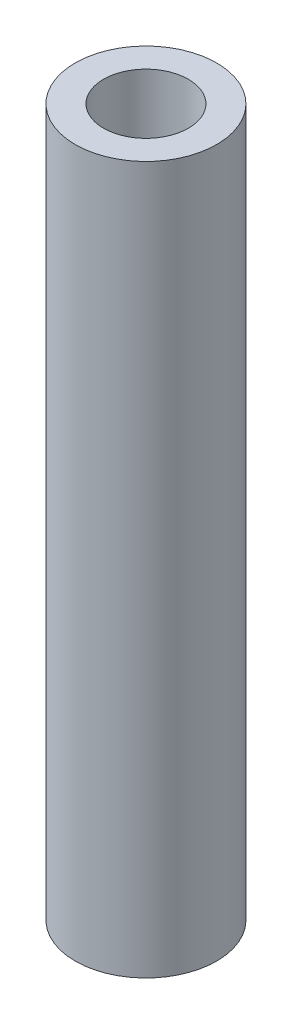
from build123d import *

# Parameters (mm, degrees)
SKETCH1_R           = 2.5
SKETCH1_R_2         = 1.5
BOSS_EXTRUDE1_DEPTH = 25
SKETCH2_R           = 1.5
SKETCH2_R_2         = 0.5
BOSS_EXTRUDE2_DEPTH = 2


with BuildPart() as part:
    # Sketch1 → Boss-Extrude1 (new body)
    with BuildSketch(Plane(origin=(0, 0, 0), x_dir=(1, 0, 0), z_dir=(0, 1, 0))):
        with Locations(Location((0, 0, 0), (0, 0, 270))):
            Circle(SKETCH1_R)
        with Locations(Location((0, 0, 0), (0, 0, 270))):
            Circle(SKETCH1_R_2, mode=Mode.SUBTRACT)
    extrude(amount=BOSS_EXTRUDE1_DEPTH)

    # Sketch2 → Boss-Extrude2 (add)
    with BuildSketch(Plane.XZ):
        with Locations(Location((0, 0, 0), (0, 0, 270))):
            Circle(SKETCH2_R)
        with Locations(Location((0, 0, 0), (0, 0, 270))):
            Circle(SKETCH2_R_2, mode=Mode.SUBTRACT)
    extrude(amount=-BOSS_EXTRUDE2_DEPTH)


solid = part.part
